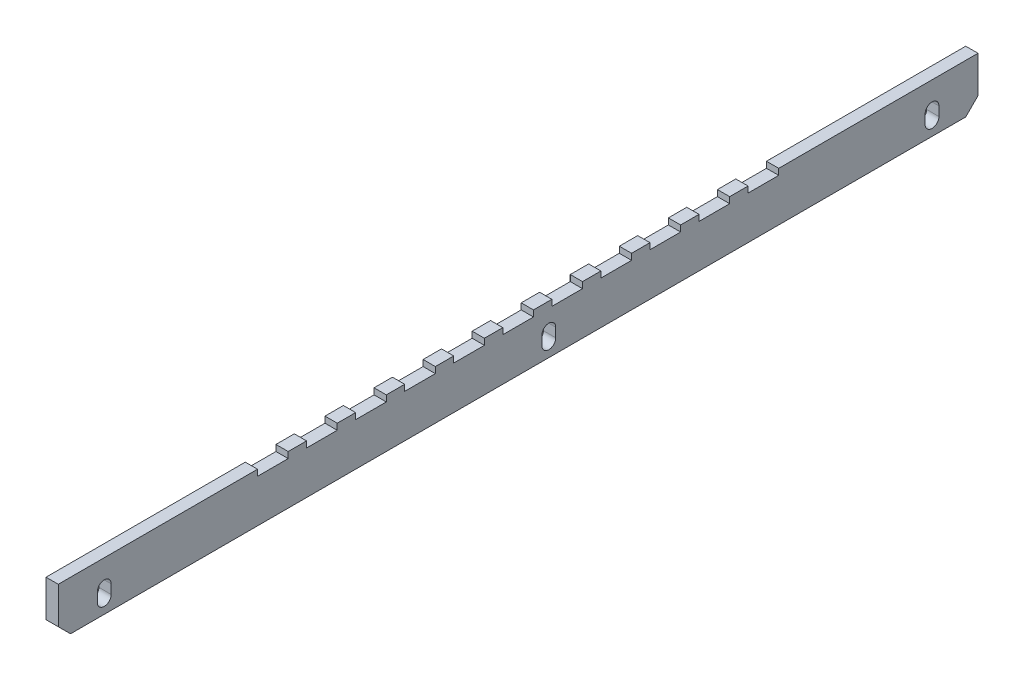
SolidWorks part; units mm, degrees
ref_plane "Front Plane" through (0, 0, 0) normal (0, 0, 1) x (1, 0, 0)
ref_plane "Top Plane" through (0, 0, 0) normal (0, 1, 0) x (1, 0, 0)
ref_plane "Right Plane" through (0, 0, 0) normal (1, 0, 0) x (0, 0, -1)
sketch "Sketch 1" plane through (0, 0, 0) normal (1, 0, 0) x (0, 0, -1)
  line L1 (-150, -8) -> (150, -8)
  line L2 (-150, -8) -> (-150, 8)
  line L3 (-150, 8) -> (150, 8)
  line L4 (150, -8) -> (150, 8)
  line L5 (-150, -8) -> (150, 8) construction
  line L6 (-150, 8) -> (150, -8) construction
  point P0 (0, 0)
  dimension "D1" = 300
  dimension "D2" = 16
extrude "Boss-Extrude 1" add sketch "Sketch 1" along normal blind 4
chamfer "Chamfer 1" distance 4 angle 45 2 edges at (2, -8, -150) (2, -8, 150)
sketch "Sketch 2" plane through (4, 0, 0) normal (1, 0, 0) x (0, 0, -1)
  line L0 (-135, -0.5) -> (-135, -3.5) construction
  line L1 (-132.75, -0.5) -> (-132.75, -3.5)
  line L2 (-137.25, -0.5) -> (-137.25, -3.5)
  line L3 (-146, -8) -> (146, -8) construction
  line L4 (-150, 8) -> (-150, -4) construction
  arc A0 (-132.75, -0.5) -> (-137.25, -0.5) centre (-135, -0.5) ccw
  arc A1 (-137.25, -3.5) -> (-132.75, -3.5) centre (-135, -3.5) ccw
  point P2 (-135, -2)
  dimension "D1" = 4.5
  dimension "D2" = 3
  dimension "D3" = 6
  dimension "D4" = 15
extrude "Cut-Extrude 1" cut sketch "Sketch 2" against normal through all
mirror "Mirror 1" about plane through (0, 0, 0) normal (0, 0, 1) of "Cut-Extrude 1"
sketch "Sketch 3" plane through (4, 0, 0) normal (1, 0, 0) x (0, 0, -1)
  line L0 (150, 8) -> (-150, 8) construction
  line L1 (-5, 10) -> (5, 10)
  line L2 (-5, 10) -> (-5, 6)
  line L3 (-5, 6) -> (5, 6)
  line L4 (5, 10) -> (5, 6)
  line L5 (-5, 10) -> (5, 6) construction
  line L6 (-5, 6) -> (5, 10) construction
  point P0 (0, 8)
  dimension "D1" = 10
  dimension "D2" = 2
extrude "Cut-Extrude 2" cut sketch "Sketch 3" against normal through all
pattern_linear "Linear Pattern 1" count 6 spacing 16 along (0, 0, -1) count 6 spacing 16 along (0, 0, 1) seed only of "Cut-Extrude 2"
sketch "Sketch 4" plane through (4, 0, 0) normal (1, 0, 0) x (0, 0, -1)
  line L0 (10, -0.5) -> (10, -3.5) construction
  line L1 (12.25, -0.5) -> (12.25, -3.5)
  line L2 (7.75, -0.5) -> (7.75, -3.5)
  line L4 (-146, -8) -> (146, -8) construction
  line L5 (150, -4) -> (150, 8) construction
  arc A0 (12.25, -0.5) -> (7.75, -0.5) centre (10, -0.5) ccw
  arc A1 (7.75, -3.5) -> (12.25, -3.5) centre (10, -3.5) ccw
  point P2 (10, -2)
  dimension "D1" = 3
  dimension "D2" = 4.5
  dimension "D3" = 140
  dimension "D4" = 4.5
extrude "Cut-Extrude 3" cut sketch "Sketch 4" against normal through all
